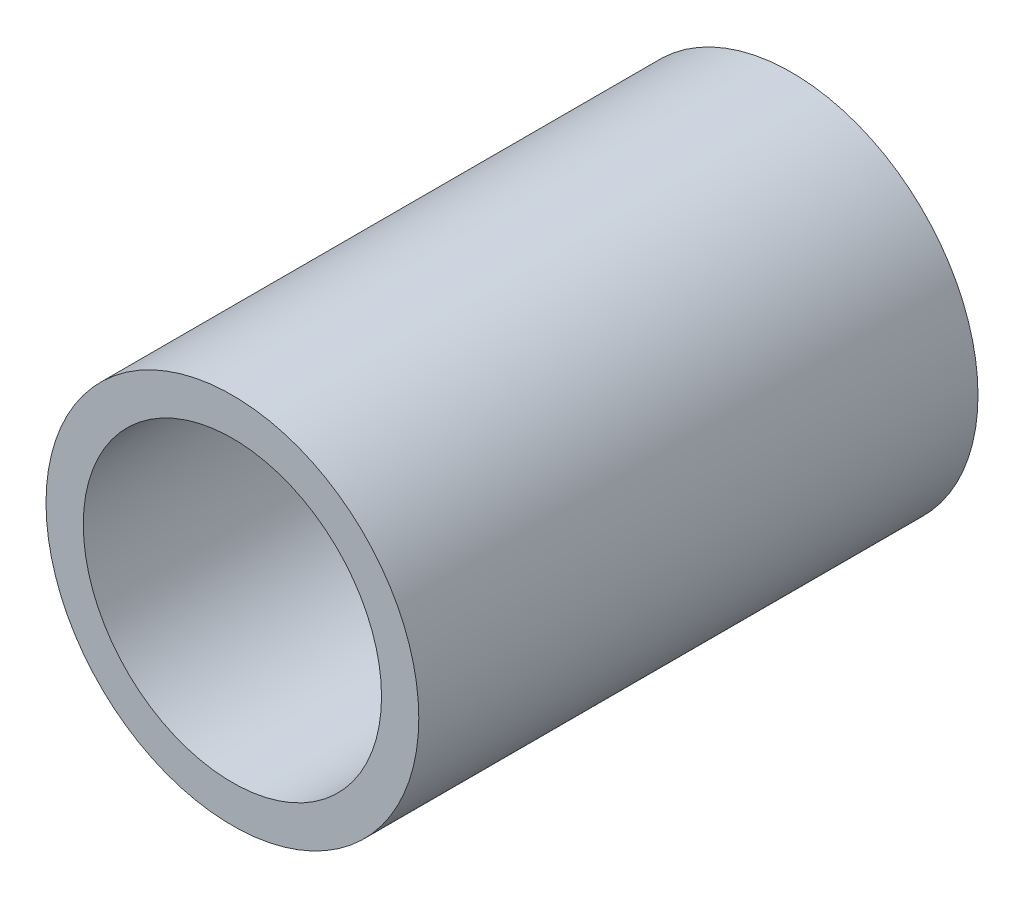
SolidWorks part; units mm, degrees
material "普通碳钢"
ref_plane "Front Plane" through (0, 0, 0) normal (0, 0, 1) x (1, 0, 0)
ref_plane "Top Plane" through (0, 0, 0) normal (0, 1, 0) x (1, 0, 0)
ref_plane "Right Plane" through (0, 0, 0) normal (1, 0, 0) x (0, 0, -1)
sketch "Sketch1" plane through (0, 0, 0) normal (0, 0, 1) x (1, 0, 0)
  circle A0 centre (0, 0) radius 40
  circle A1 centre (0, 0) radius 50
  dimension "D1" = 100
  dimension "D2" = 80
extrude "Boss-Extrude1" add sketch "Sketch1" along normal blind 150
sketch "Sketch2" plane through (0, 0, 0) normal (0, 0, -1) x (-1, 0, 0)
  line L0 (0, 0) -> (-50, 0) construction
  line L1 (0, 0) -> (0, 50) construction
  circle A0 centre (0, 0) radius 50 construction
